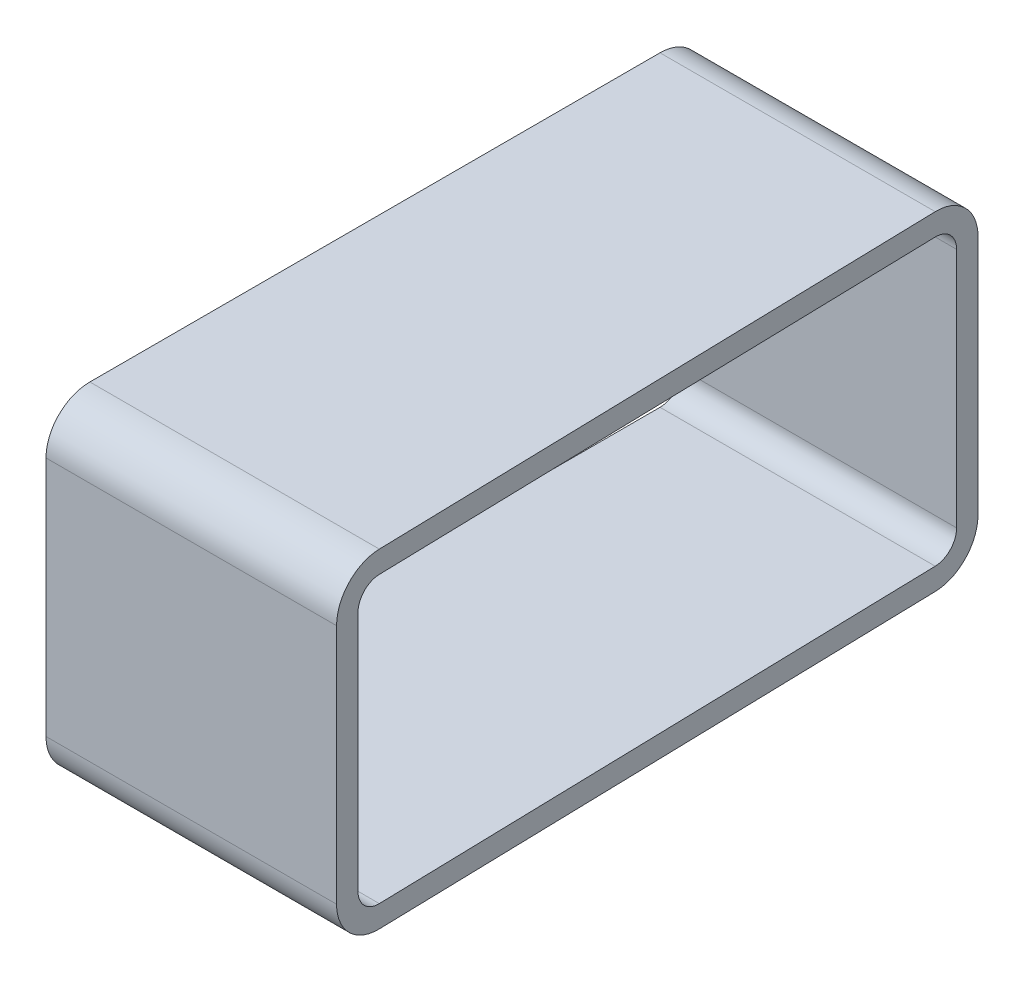
from build123d import *

# Parameters (mm, degrees)
GB_6728_1986_RECTANGULAR_HOLLOW_SECTION_DEPTH = 53
CUT_EXTRUDE1_DEPTH                            = 101.04498988
CUT_EXTRUDE1_DEPTH_BACK                       = 101.04498988


with BuildPart() as part:
    # Sketch1 → GB/6728-1986 rectangular hollow section 120 X 60 X 4(1) (new body)
    with BuildSketch(Plane.YZ):
        with BuildLine():
            Line((-22, -60), (22, -60))
            ThreePointArc((22, -60), (27.656854249, -57.656854249), (30, -52))
            Line((30, -52), (30, 52))
            ThreePointArc((30, 52), (27.656854249, 57.656854249), (22, 60))
            Line((22, 60), (-22, 60))
            ThreePointArc((-22, 60), (-27.656854249, 57.656854249), (-30, 52))
            Line((-30, 52), (-30, -52))
            ThreePointArc((-30, -52), (-27.656854249, -57.656854249), (-22, -60))
        make_face()
        with BuildLine():
            Line((-22, -56), (22, -56))
            ThreePointArc((22, -56), (24.828427125, -54.828427125), (26, -52))
            Line((26, -52), (26, 52))
            ThreePointArc((26, 52), (24.828427125, 54.828427125), (22, 56))
            Line((22, 56), (-22, 56))
            ThreePointArc((-22, 56), (-24.828427125, 54.828427125), (-26, 52))
            Line((-26, 52), (-26, -52))
            ThreePointArc((-26, -52), (-24.828427125, -54.828427125), (-22, -56))
        make_face(mode=Mode.SUBTRACT)
    extrude(amount=GB_6728_1986_RECTANGULAR_HOLLOW_SECTION_DEPTH)

    # Sketch3 → Cut-Extrude1 (cut, two sides: drawn at the far end of the back side and taken through both)
    with BuildSketch(Plane.XZ.offset(30).offset(-CUT_EXTRUDE1_DEPTH_BACK)):
        Polygon((53, 60), (50, -60), (53, -60), align=None)
    extrude(amount=CUT_EXTRUDE1_DEPTH + CUT_EXTRUDE1_DEPTH_BACK, mode=Mode.SUBTRACT)


solid = part.part
